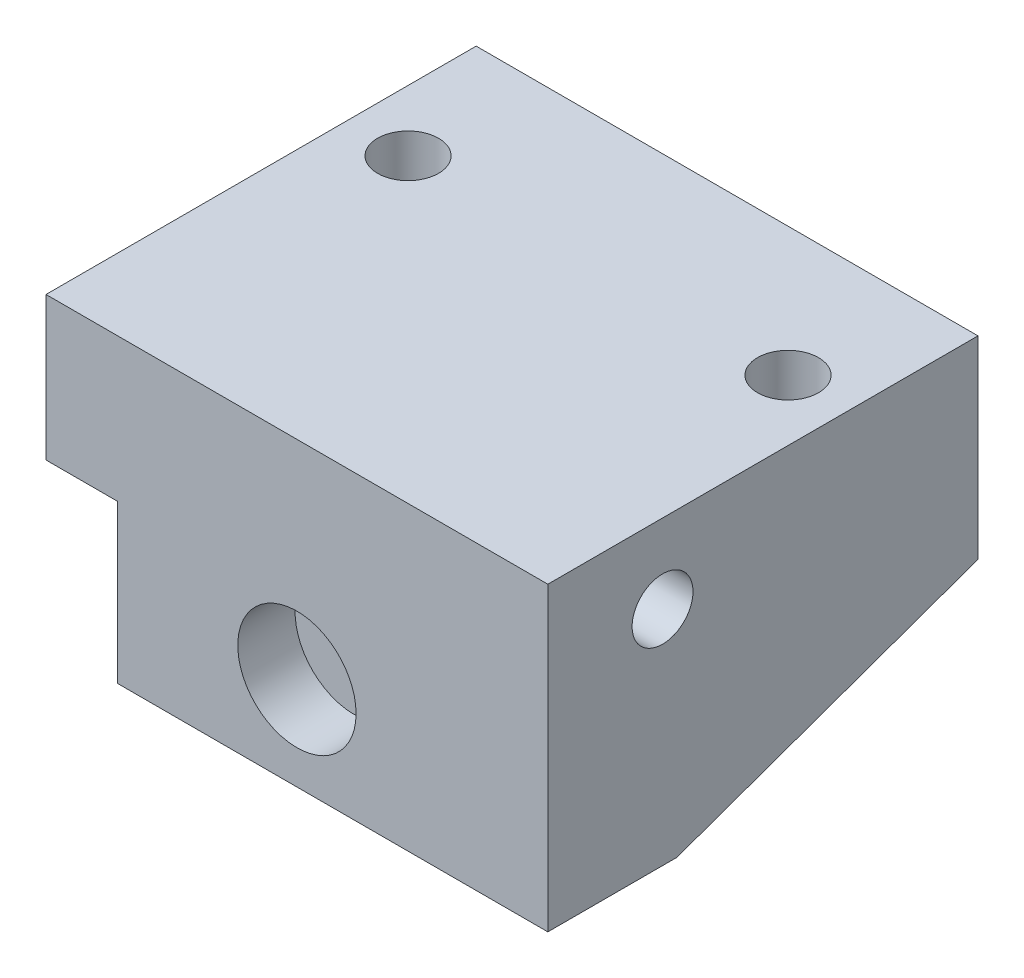
SolidWorks part; units mm, degrees
other "Markup1"
sketch "草图9" plane through (-35, 20, -30) normal (0, 1, 0) x (-1, 0, 0)
ref_plane "Front Plane" through (0, 0, 0) normal (0, 0, 1) x (1, 0, 0)
ref_plane "Top Plane" through (0, 0, 0) normal (0, 1, 0) x (1, 0, 0)
ref_plane "Right Plane" through (0, 0, 0) normal (1, 0, 0) x (0, 0, -1)
sketch "Sketch1" plane through (0, 0, 0) normal (0, 1, 0) x (1, 0, 0)
  line L1 (-35, 30) -> (35, 30)
  line L2 (-35, 30) -> (-35, -30)
  line L3 (-35, -30) -> (35, -30)
  line L4 (35, 30) -> (35, -30)
  line L5 (-35, 30) -> (35, -30) construction
  line L6 (-35, -30) -> (35, 30) construction
  point P0 (0, 0)
  dimension "D1" = 70
  dimension "D2" = 60
extrude "Boss-Extrude1" add sketch "Sketch1" along normal blind 20
sketch "Sketch2" plane through (35, 0, 0) normal (1, 0, 0) x (0, 0, -1)
  line L0 (30, 20) -> (30, 0)
  line L1 (30, 0) -> (30, -7)
  line L2 (30, -7) -> (-12, -22)
  line L3 (-12, -22) -> (-30, -22)
  line L4 (-30, -22) -> (-30, 20)
  line L5 (-30, 20) -> (30, 20)
  dimension "D1" = 42
  dimension "D2" = 18
  dimension "D3" = 27
extrude "Boss-Extrude2" add sketch "Sketch2" against normal blind 60
sketch "Sketch5" plane through (-35, 0, 0) normal (-1, 0, 0) x (0, 0, 1)
  line L0 (30, 20) -> (30, 0) construction
  line L1 (-30, 20) -> (30, 20) construction
  circle A1 centre (14, 9) radius 4.25
  dimension "D1" = 16
  dimension "D3" = 8.5
  dimension "D2" = 11
extrude "Cut-Extrude3" cut sketch "Sketch5" against normal blind 131
sketch "Sketch7" plane through (0, 20, 0) normal (0, 1, 0) x (1, 0, 0)
  line L1 (35, 30) -> (-35, 30) construction
  line L2 (0, 10) -> (0, -8.5493) construction
  line L3 (-35, 30) -> (-35, -30) construction
  circle A1 centre (26.5, 12) radius 4.25
  circle A2 centre (-26.5, 12) radius 4.25
  dimension "D1" = 8.5
  dimension "D2" = 8.5
  dimension "D3" = 18
extrude "Cut-Extrude4" cut sketch "Sketch7" against normal blind 91
sketch "Sketch8" plane through (0, 0, 30) normal (0, 0, 1) x (1, 0, 0)
  line L0 (0, 22.3133) -> (0, -18.434) construction
  line L1 (-25, -22) -> (35, -22) construction
  circle A0 centre (0, -9) radius 8.25
  dimension "D1" = 16.5
  dimension "D2" = 13
extrude "Cut-Extrude5" cut sketch "Sketch8" against normal blind 8
